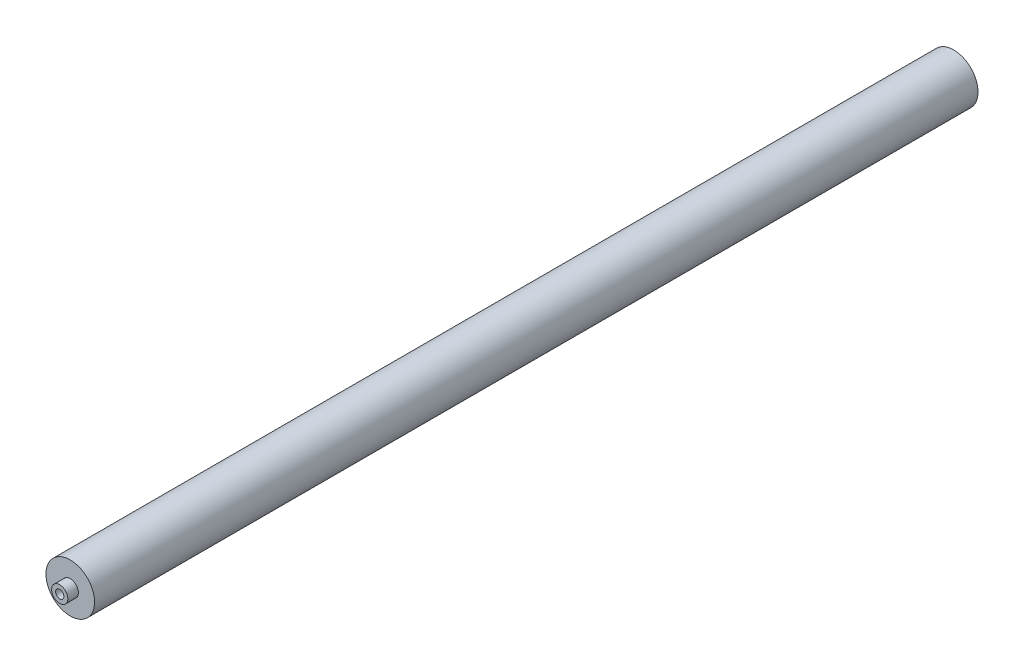
SolidWorks part; units mm, degrees
material "1023 碳钢板 (SS)"
ref_plane "Front Plane" through (0, 0, 0) normal (0, 0, 1) x (1, 0, 0)
ref_plane "Top Plane" through (0, 0, 0) normal (0, 1, 0) x (1, 0, 0)
ref_plane "Right Plane" through (0, 0, 0) normal (1, 0, 0) x (0, 0, -1)
sketch "Sketch1" plane through (0, 0, 0) normal (0, 0, 1) x (1, 0, 0)
  circle A0 centre (0, 0) radius 30
  dimension "D1" = 60
extrude "Boss-Extrude1" add sketch "Sketch1" along normal blind 1090
sketch "Sketch2" plane through (0, 0, 1090) normal (0, 0, 1) x (1, 0, 0)
  circle A0 centre (0, 0) radius 10
  dimension "D1" = 20
extrude "Boss-Extrude2" add sketch "Sketch2" along normal blind 13
sketch "Sketch3" plane through (0, 0, 0) normal (0, 0, -1) x (-1, 0, 0)
  circle A0 centre (0, 0) radius 10
  dimension "D1" = 20
extrude "Boss-Extrude3" add sketch "Sketch3" along normal blind 13
hole_wizard "M12 Tapped Hole1" positions "Sketch4" profile "Sketch5" tap size "M12" standard "ISO"
sketch "Sketch4" plane through (0, 0, -13) normal (0, 0, -1) x (-1, 0, 0)
  point P0 (0, 0)
sketch "Sketch5" plane through (0, 0, -13) normal (1, 0, 0) x (0, 1, 0)
  line L0 (0, 0) -> (0, 28.3144)
  line L1 (0, 28.3144) -> (5.1, 25.25)
  line L2 (5.1, 25.25) -> (5.1, 0)
  line L5 (5.1, 0) -> (0, 0)
  line L10 (0, 28.3144) -> (-5.1, 25.25) construction
  line L11 (0, -6.35) -> (0, 107.95) construction
  dimension "螺纹孔钻头直径" = 10.2
  dimension "螺纹孔钻头深度" = 25.25
  dimension "导头角度" = 118
cosmetic thread "Hole Thread Line1" parameters "D1"=20, "D2"=12
hole_wizard "M12 Tapped Hole2" positions "Sketch6" profile "Sketch7" tap size "M12" standard "ISO"
sketch "Sketch6" plane through (0, 0, 1103) normal (0, 0, 1) x (1, 0, 0)
  point P0 (0, 0)
sketch "Sketch7" plane through (0, 0, 1103) normal (1, 0, 0) x (0, -1, 0)
  line L0 (0, 0) -> (0, 28.3144)
  line L1 (0, 28.3144) -> (5.1, 25.25)
  line L2 (5.1, 25.25) -> (5.1, 0)
  line L5 (5.1, 0) -> (0, 0)
  line L10 (0, 28.3144) -> (-5.1, 25.25) construction
  line L11 (0, -6.35) -> (0, 107.95) construction
  dimension "螺纹孔钻头直径" = 10.2
  dimension "螺纹孔钻头深度" = 25.25
  dimension "导头角度" = 118
cosmetic thread "Hole Thread Line2" parameters "D1"=20, "D2"=12
